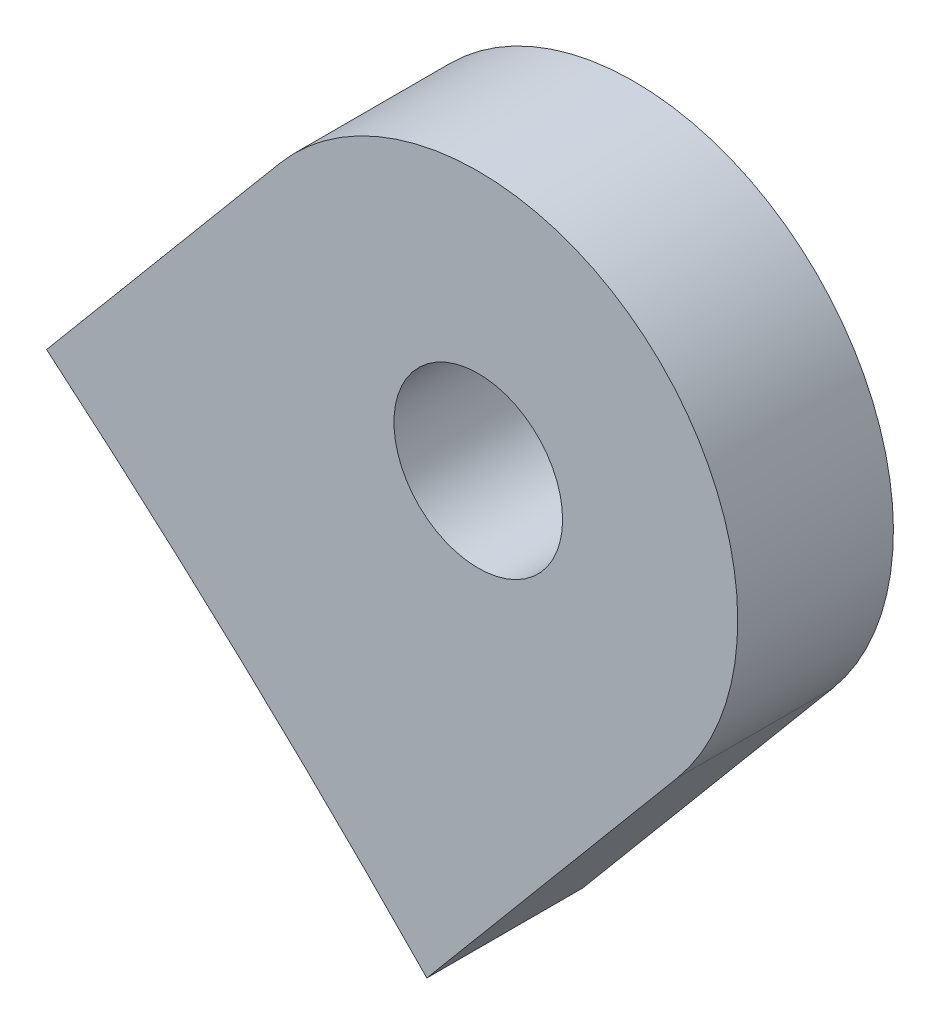
from build123d import *

# Parameters (mm, degrees)
SKETCH1_R           = 6.499999992
BOSS_EXTRUDE1_DEPTH = 6


with BuildPart() as part:
    # Sketch1 → Boss-Extrude1 (new, symmetric)
    with BuildSketch(Plane.XY):
        with BuildLine():
            Line((249.080198754, 296.842221709), (267.033227589, 318.237808321))
            ThreePointArc((267.033227589, 318.237808321), (295.209868645, 320.702944991), (297.675005315, 292.526303935))
            Line((297.675005315, 292.526303935), (278.391377025, 269.544970642))
            ThreePointArc((278.391377025, 269.544970642), (264.088717655, 283.572564272), (249.080198754, 296.842221709))
        make_face()
        with Locations((282.354116452, 305.382056128)):
            Circle(SKETCH1_R, mode=Mode.SUBTRACT)
    extrude(amount=BOSS_EXTRUDE1_DEPTH, both=True)


solid = part.part
